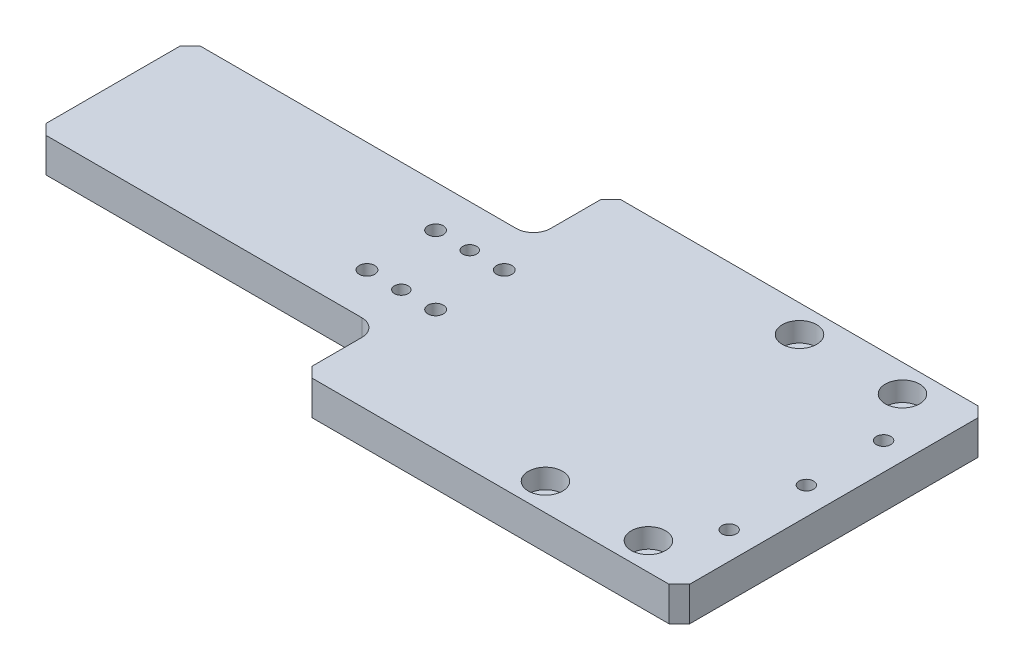
from build123d import *

# Parameters (mm, degrees)
SKETCH_1_W                = 210
SKETCH_1_H                = 90
EXTRUDE_1_DEPTH           = 10
CHAMFER_1_SIZE            = 3
HOLE_WIZARD_2_D           = 5.5
HOLE_WIZARD_2_DEPTH       = 10.1
HOLE_WIZARD_2_CBORE_D     = 10
HOLE_WIZARD_2_CBORE_DEPTH = 5.7
HOLE_WIZARD_2_TIP         = 1.652366702
SKETCH_4_W                = 100
SKETCH_4_H                = 22.5
CUT_EXTRUDE_1_DEPTH       = 20
CHAMFER_2_SIZE            = 3
FILLET_1_R                = 5
HOLE_WIZARD_0_D           = 4.5
HOLE_WIZARD_0_DEPTH       = 25
HOLE_WIZARD_0_CBORE_D     = 8
HOLE_WIZARD_0_CBORE_DEPTH = 4.6
HOLE_WIZARD_0_TIP         = 1.351936393
MM_0_D                    = 4
MM_0_DEPTH                = 25
MM_0_TIP                  = 1.201721238
HOLE_WIZARD_M5_1_D        = 4.2
HOLE_WIZARD_M5_1_DEPTH    = 12.4
HOLE_WIZARD_M5_1_TIP      = 1.2618073


with BuildPart() as part:
    # 草图1 → 凸台-拉伸1 (new body)
    with BuildSketch(Plane(origin=(0, 0, 0), x_dir=(1, 0, 0), z_dir=(0, 1, 0))):
        Rectangle(SKETCH_1_W, SKETCH_1_H)
    extrude(amount=EXTRUDE_1_DEPTH)

    # 倒角1
    chamfer_1_edges = [part.edges().sort_by_distance(p)[0] for p in [
        (105, 5, 45),
        (-105, 5, 45),
        (-105, 5, -45),
        (105, 5, -45),
    ]]
    chamfer(chamfer_1_edges, length=CHAMFER_1_SIZE)

    # 打孔尺寸(%根据)内六角圆柱头螺钉的类型2
    with Locations(Plane(origin=(0, 10, 0), x_dir=(1, 0, 0), z_dir=(0, 1, 0))):
        with Locations((58, -37), (58, 37), (88, 37), (88, -37)):
            CounterBoreHole(HOLE_WIZARD_2_D / 2, HOLE_WIZARD_2_CBORE_D / 2, HOLE_WIZARD_2_CBORE_DEPTH, depth=HOLE_WIZARD_2_DEPTH)
            with Locations((0, 0, -(HOLE_WIZARD_2_DEPTH + HOLE_WIZARD_2_TIP / 2))):  # 118° drill point
                Cone(0, HOLE_WIZARD_2_D / 2, HOLE_WIZARD_2_TIP, mode=Mode.SUBTRACT)

    # 草图4 → 切除-拉伸1 (cut)
    with BuildSketch(Plane(origin=(0, 10, 0), x_dir=(1, 0, 0), z_dir=(0, 1, 0))):
        with Locations((-55, -33.75)):
            Rectangle(SKETCH_4_W, SKETCH_4_H)
        with Locations((-55, 33.75)):
            Rectangle(SKETCH_4_W, SKETCH_4_H)
    extrude(amount=-CUT_EXTRUDE_1_DEPTH, mode=Mode.SUBTRACT)

    # 倒角2
    chamfer_2_edges = [part.edges().sort_by_distance(p)[0] for p in [
        (-105, 5, 22.5),
        (-5, 5, 45),
        (-5, 5, -45),
        (-105, 5, -22.5),
    ]]
    chamfer(chamfer_2_edges, length=CHAMFER_2_SIZE)

    # 圆角1
    fillet_1_edges = [part.edges().sort_by_distance(p)[0] for p in [
        (-5, 5, 22.5),
        (-5, 5, -22.5),
    ]]
    fillet(fillet_1_edges, radius=FILLET_1_R)

    # 打孔尺寸(%根据)内六角圆柱头螺钉的类型0
    with Locations(Plane(origin=(0, 0, 0), x_dir=(-1, 0, 0), z_dir=(0, -1, 0))):
        with Locations((21.3, 10.3), (21.3, -9.7), (1.3, 10.3), (1.3, -9.7)):
            CounterBoreHole(HOLE_WIZARD_0_D / 2, HOLE_WIZARD_0_CBORE_D / 2, HOLE_WIZARD_0_CBORE_DEPTH, depth=HOLE_WIZARD_0_DEPTH)
            with Locations((0, 0, -(HOLE_WIZARD_0_DEPTH + HOLE_WIZARD_0_TIP / 2))):  # 118° drill point
                Cone(0, HOLE_WIZARD_0_D / 2, HOLE_WIZARD_0_TIP, mode=Mode.SUBTRACT)

    # 大小mm 暗销孔0
    with Locations(Plane(origin=(0, 0, 0), x_dir=(-1, 0, 0), z_dir=(0, -1, 0))):
        with Locations((11.3, -9.7), (11.3, 10.231708661)):
            Hole(MM_0_D / 2, depth=MM_0_DEPTH)
            with Locations((0, 0, -(MM_0_DEPTH + MM_0_TIP / 2))):  # 118° drill point
                Cone(0, MM_0_D / 2, MM_0_TIP, mode=Mode.SUBTRACT)

    # M5 螺纹孔1
    with Locations(Plane(origin=(0, 10, 0), x_dir=(1, 0, 0), z_dir=(0, 1, 0))):
        with Locations((97, -22.5), (97, 0), (97, 22.5)):
            Hole(HOLE_WIZARD_M5_1_D / 2, depth=HOLE_WIZARD_M5_1_DEPTH)
            with Locations((0, 0, -(HOLE_WIZARD_M5_1_DEPTH + HOLE_WIZARD_M5_1_TIP / 2))):  # 118° drill point
                Cone(0, HOLE_WIZARD_M5_1_D / 2, HOLE_WIZARD_M5_1_TIP, mode=Mode.SUBTRACT)


solid = part.part
